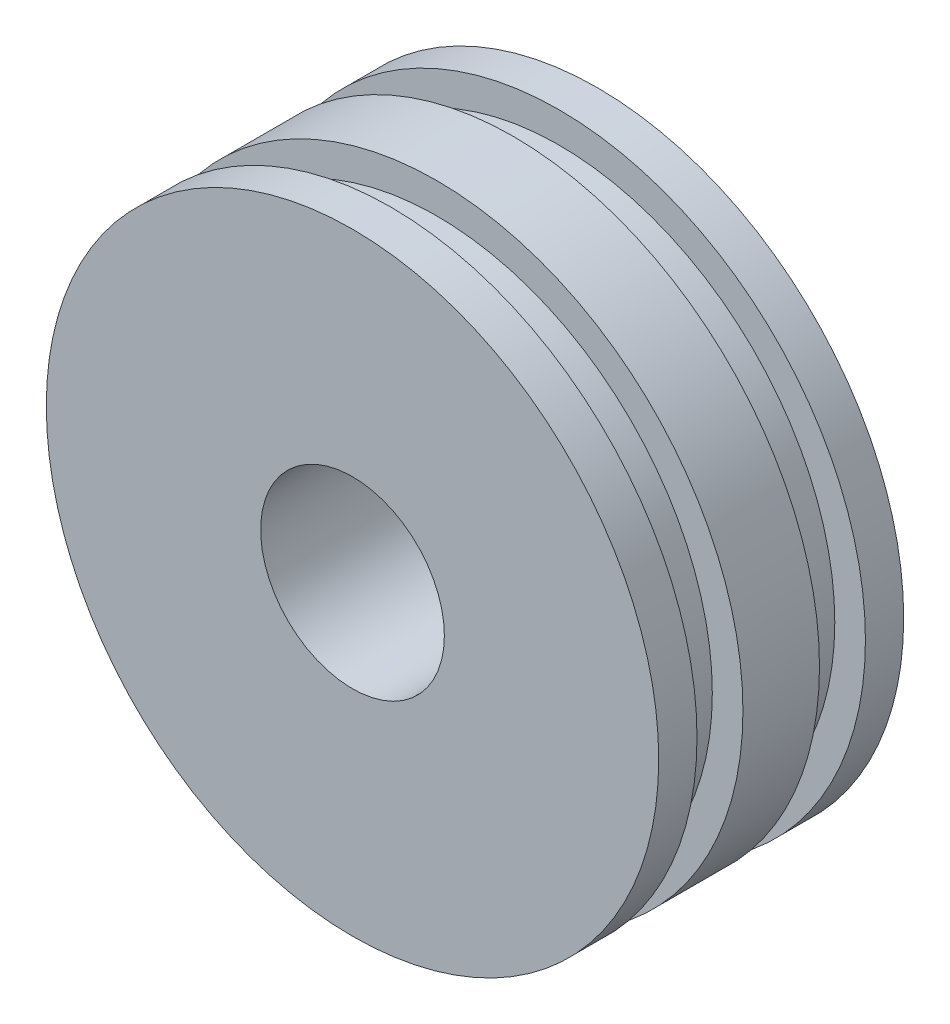
from build123d import *

# Parameters (mm, degrees)
SKETCH_1_R          = 100
SKETCH_1_R_2        = 30
EXTRUDE_1_DEPTH     = 40
SKETCH_2_R          = 100
SKETCH_2_R_2        = 90
CUT_EXTRUDE_1_DEPTH = 7.5


with BuildPart() as part:
    # 草图1 → 凸台-拉伸1 (new, symmetric)
    with BuildSketch(Plane.XY):
        Circle(SKETCH_1_R)
        Circle(SKETCH_1_R_2, mode=Mode.SUBTRACT)
    extrude(amount=EXTRUDE_1_DEPTH, both=True)

    # 草图2 → 切除-拉伸1 (cut, symmetric)
    with BuildSketch(Plane.XY.offset(20)):
        Circle(SKETCH_2_R)
        Circle(SKETCH_2_R_2, mode=Mode.SUBTRACT)
    cut_extrude_1 = extrude(amount=CUT_EXTRUDE_1_DEPTH, both=True, mode=Mode.SUBTRACT)

    # 镜向1: 切除-拉伸1 across plane
    add(cut_extrude_1.mirror(Plane.XY), mode=Mode.SUBTRACT)


solid = part.part
